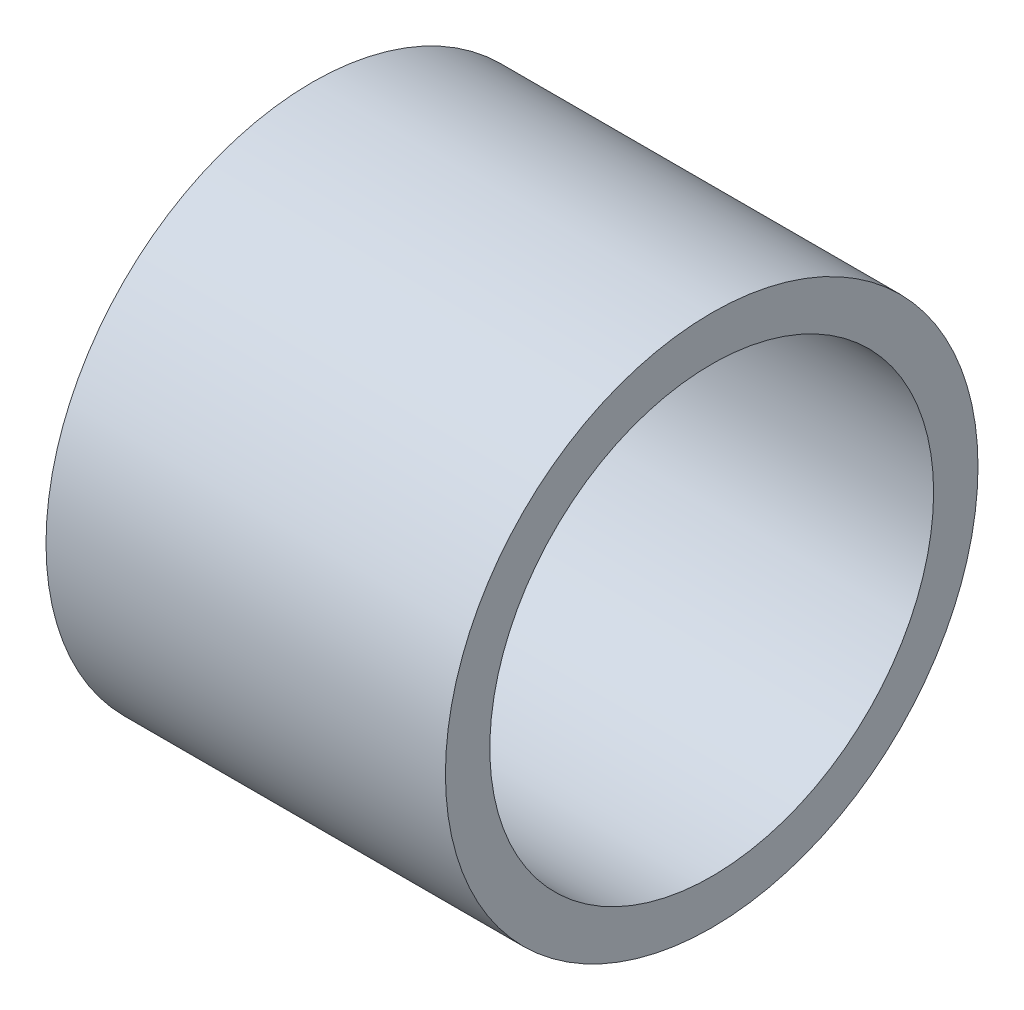
from build123d import *

# Parameters (mm, degrees)
SKETCH1_R           = 12
SKETCH1_R_2         = 10
BOSS_EXTRUDE1_DEPTH = 18


with BuildPart() as part:
    # Sketch1 → Boss-Extrude1 (new body)
    with BuildSketch(Plane(origin=(0, 0, 0), x_dir=(0, 0, -1), z_dir=(1, 0, 0))):
        Circle(SKETCH1_R)
        Circle(SKETCH1_R_2, mode=Mode.SUBTRACT)
    extrude(amount=BOSS_EXTRUDE1_DEPTH)


solid = part.part
